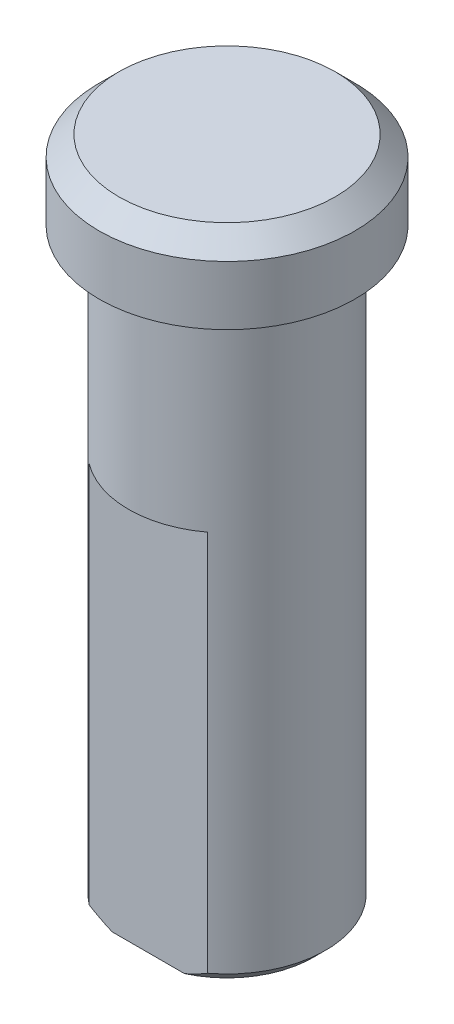
SolidWorks part; units mm, degrees
ref_plane "Front Plane" through (0, 0, 0) normal (0, 0, 1) x (1, 0, 0)
ref_plane "Top Plane" through (0, 0, 0) normal (0, 1, 0) x (1, 0, 0)
ref_plane "Right Plane" through (0, 0, 0) normal (1, 0, 0) x (0, 0, -1)
sketch "Sketch1" plane through (0, 0, 0) normal (0, 1, 0) x (1, 0, 0)
  circle A0 centre (0, 0) radius 2.5
  dimension "D1" = 5
extrude "Boss-Extrude1" add sketch "Sketch1" along normal blind 15
sketch "Sketch2" plane through (0, 15, 0) normal (0, 1, 0) x (1, 0, 0)
  circle A0 centre (0, 0) radius 3.25
  dimension "D1" = 6.5
extrude "Boss-Extrude2" add sketch "Sketch2" along normal blind 2
chamfer "Chamfer1" distance 0.5 angle 45 1 edges at (0, 17, 3.25)
chamfer "Chamfer2" distance 0.3 angle 45 1 edges at (0, 0, 2.5)
sketch "Sketch3" plane through (0, 0, 0) normal (0, -1, 0) x (1, 0, 0)
  line L0 (0, 0) -> (0, 50000) construction
  line L2 (-2.9571, 3) -> (2.9571, 3)
  line L3 (-2.9571, 3) -> (-2.9571, 2)
  line L4 (-2.9571, 2) -> (2.9571, 2)
  line L5 (2.9571, 3) -> (2.9571, 2)
  line L6 (-2.9571, 3) -> (2.9571, 2) construction
  line L7 (-2.9571, 2) -> (2.9571, 3) construction
  circle A0 centre (0, 0) radius 2.5 construction
  point P3 (0, 2.5)
  dimension "D1" = 2
extrude "Cut-Extrude1" cut sketch "Sketch3" against normal blind 10
